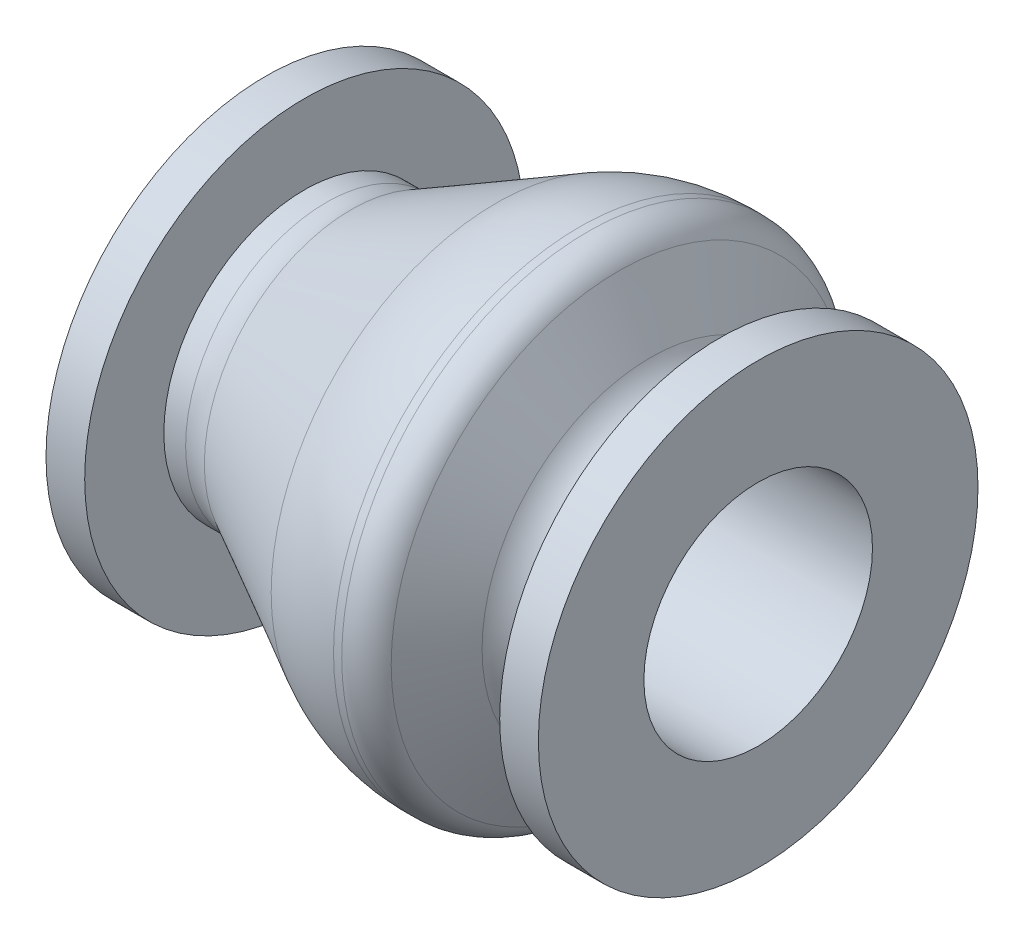
from build123d import *


with BuildPart() as part:
    # Sketch1 → Revolve1 (revolve)
    with BuildSketch(Plane.XY, mode=Mode.PRIVATE) as revolve1_sk:
        with BuildLine():
            Line((0, 65), (0, 125))
            Line((0, 125), (22, 125))
            Line((22, 125), (22, 80))
            Line((22, 80), (34.398449785, 80))
            ThreePointArc((34.398449785, 80), (41.732480398, 80.910276815), (48.621444476, 83.585867002))
            Line((48.621444476, 83.585867002), (130.980482924, 127.933041551))
            ThreePointArc((130.980482924, 127.933041551), (153.943696517, 136.851675508), (178.390465228, 139.885931559))
            Line((178.390465228, 139.885931559), (183.05792065, 139.885931559))
            ThreePointArc((183.05792065, 139.885931559), (193.313652481, 137.056253763), (200.667342649, 129.36792802))
            Line((200.667342649, 129.36792802), (218.75476257, 95.777005309))
            ThreePointArc((218.75476257, 95.777005309), (229.785297821, 84.244516693), (245.168895567, 80))
            Line((245.168895567, 80), (258, 80))
            Line((258, 80), (258, 125))
            Line((258, 125), (280, 125))
            Line((280, 125), (280, 65))
            Line((280, 65), (0, 65))
        make_face()
    revolve(revolve1_sk.sketch.rotate(Axis((0, 0, 0), (1, 0, 0)), 90), axis=Axis((0, 0, 0), (1, 0, 0)))


solid = part.part
